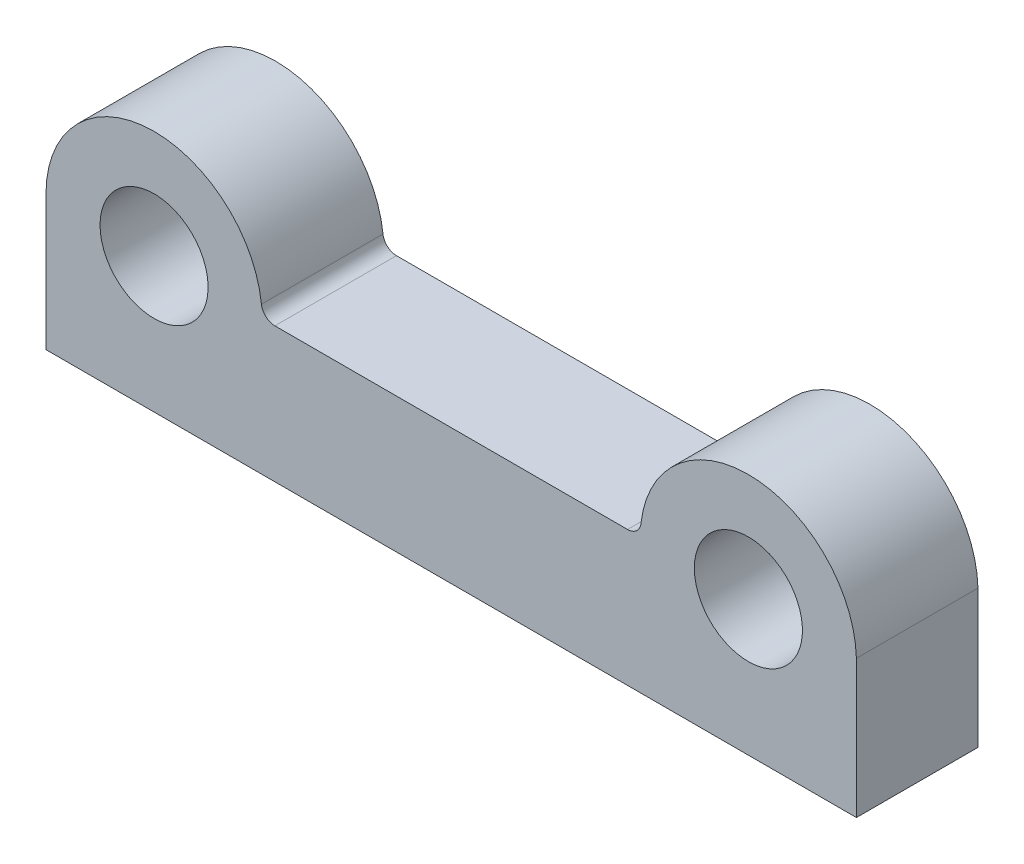
from build123d import *

# Parameters (mm, degrees)
SKETCH1_R           = 40
BOSS_EXTRUDE2_DEPTH = 90


with BuildPart() as part:
    # Sketch1 → Boss-Extrude2 (new body)
    with BuildSketch(Plane.XY):
        with BuildLine():
            ThreePointArc((-140.4953608, 8.888888889), (-224.451340472, 79.876063799), (-300, 0))
            Line((-300, 0), (-300, -100))
            Line((-300, -100), (300, -100))
            Line((300, -100), (299.972882257, -2.08281146))
            Line((299.972882257, -2.08281146), (299.971716338, 2.127107427))
            ThreePointArc((299.971716338, 2.127107427), (223.388947093, 79.928186753), (140.4953608, 8.888888889))
            ThreePointArc((140.4953608, 8.888888889), (137.223947567, 2.546440075), (130.5572809, 0))
            Line((130.5572809, 0), (-130.5572809, 0))
            ThreePointArc((-130.5572809, 0), (-137.223947567, 2.546440075), (-140.4953608, 8.888888889))
        make_face()
        with Locations(Location((-220, 0, 0), (0, 0, 180))):
            Circle(SKETCH1_R, mode=Mode.SUBTRACT)
        with Locations(Location((220, 0, 0), (0, 0, 180))):
            Circle(SKETCH1_R, mode=Mode.SUBTRACT)
    extrude(amount=BOSS_EXTRUDE2_DEPTH)


solid = part.part
